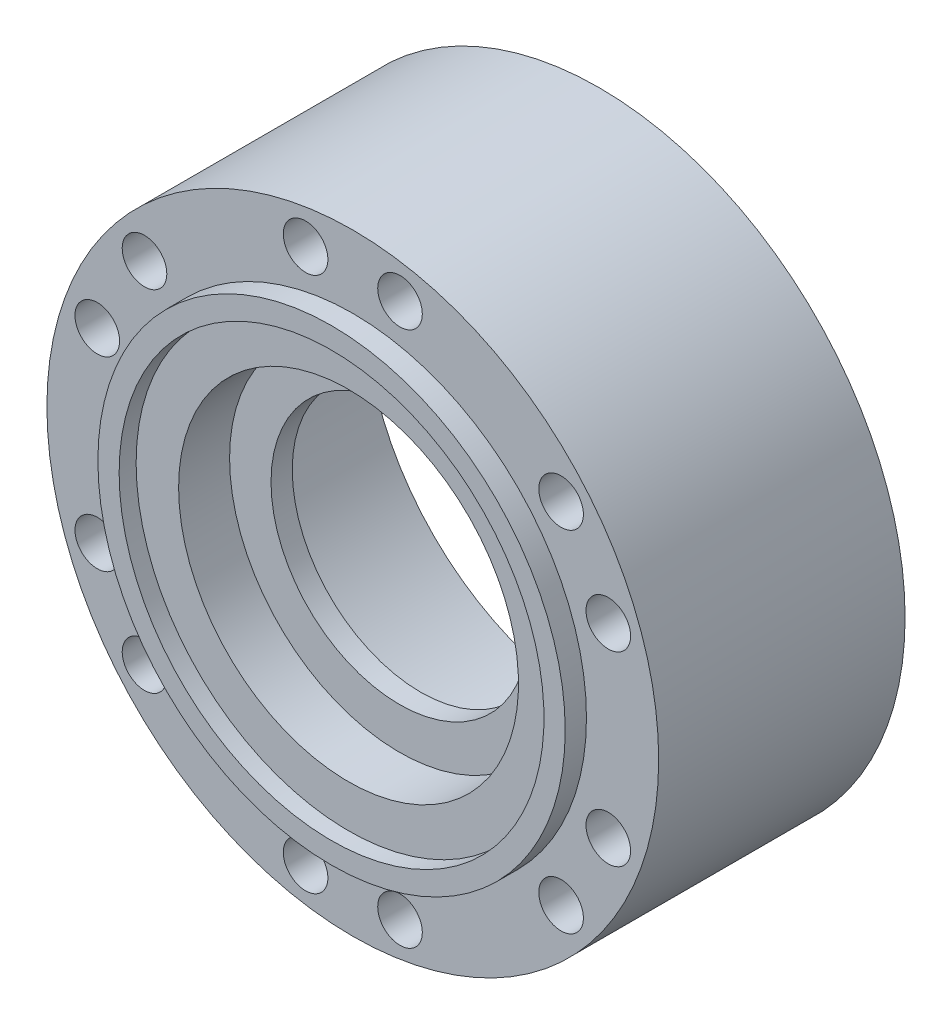
from build123d import *

# Parameters (mm, degrees)
SKETCH1_R                    = 72
BOSS_EXTRUDE1_DEPTH          = 58
SKETCH2_R                    = 55
BOSS_EXTRUDE2_DEPTH          = 5
F_10_5_10_5_DIAMETER_HOLE1_D = 10.5
SKETCH5_R                    = 55
CUT_EXTRUDE1_DEPTH           = 42
SKETCH6_R                    = 30.25
CUT_EXTRUDE2_DEPTH           = 5
SKETCH7_R                    = 40
CUT_EXTRUDE3_DEPTH           = 12
SKETCH9_R                    = 50
CUT_EXTRUDE4_DEPTH           = 4


with BuildPart() as part:
    # Sketch1 → Boss-Extrude1 (new body)
    with BuildSketch(Plane.XY):
        with Locations(Location((0, 0, 0), (0, 0, 180))):
            Circle(SKETCH1_R)
    extrude(amount=BOSS_EXTRUDE1_DEPTH)

    # Sketch2 → Boss-Extrude2 (add)
    with BuildSketch(Plane.XY.offset(58)):
        Circle(SKETCH2_R)
    extrude(amount=BOSS_EXTRUDE2_DEPTH)

    # Ø10.5 (10.5) Diameter Hole1 (through all)
    with Locations(Plane(origin=(0, 0, 0), x_dir=(-1, 0, 0), z_dir=(0, 0, -1))):
        with Locations((-11.113483371, 63.027696193), (11.113483371, 63.027696193), (49.02684436, 41.13840702), (60.14032773, 21.889289173), (60.14032773, -21.889289173), (49.02684436, -41.13840702), (11.113483371, -63.027696193), (-11.113483371, -63.027696193), (-49.02684436, -41.13840702), (-60.14032773, -21.889289173), (-60.14032773, 21.889289173), (-49.02684436, 41.13840702)):
            Hole(F_10_5_10_5_DIAMETER_HOLE1_D / 2)

    # Sketch5 → Cut-Extrude1 (cut)
    with BuildSketch(Plane(origin=(0, 0, 0), x_dir=(-1, 0, 0), z_dir=(0, 0, -1))):
        with Locations(Location((0, 0, 0), (0, 0, 180))):
            Circle(SKETCH5_R)
    extrude(amount=-CUT_EXTRUDE1_DEPTH, mode=Mode.SUBTRACT)

    # Sketch6 → Cut-Extrude2 (cut)
    with BuildSketch(Plane(origin=(0, 0, 42), x_dir=(-1, 0, 0), z_dir=(0, 0, -1))):
        Circle(SKETCH6_R)
    extrude(amount=-CUT_EXTRUDE2_DEPTH, mode=Mode.SUBTRACT)

    # Sketch7 → Cut-Extrude3 (cut)
    with BuildSketch(Plane(origin=(0, 0, 47), x_dir=(-1, 0, 0), z_dir=(0, 0, -1))):
        Circle(SKETCH7_R)
    extrude(amount=-CUT_EXTRUDE3_DEPTH, mode=Mode.SUBTRACT)

    # Sketch9 → Cut-Extrude4 (cut)
    with BuildSketch(Plane(origin=(0, 0, 59), x_dir=(-1, 0, 0), z_dir=(0, 0, -1))):
        Circle(SKETCH9_R)
    extrude(amount=-CUT_EXTRUDE4_DEPTH, mode=Mode.SUBTRACT)


solid = part.part
